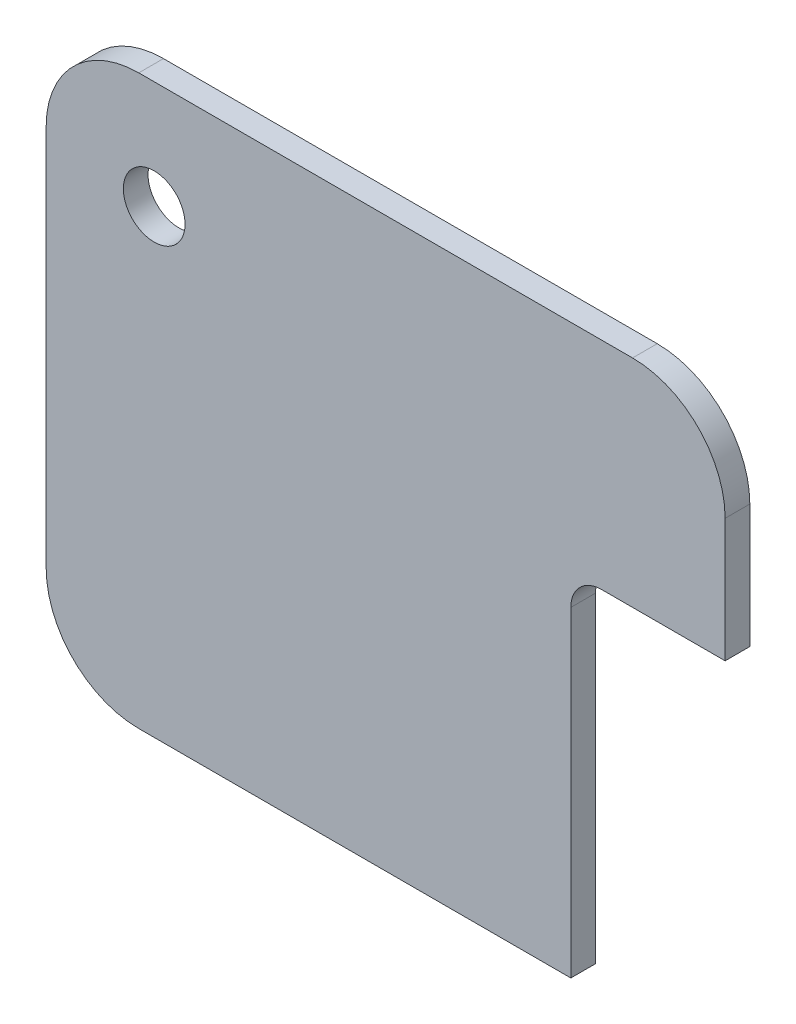
from build123d import *

# Parameters (mm, degrees)
SKETCH_1_R      = 10
EXTRUDE_1_DEPTH = 8


with BuildPart() as part:
    # 草图1 → 凸台-拉伸1 (new body)
    with BuildSketch(Plane.XY):
        with BuildLine():
            Line((0, 30), (0, 154))
            ThreePointArc((0, 154), (8.786796564, 175.213203436), (30, 184))
            Line((30, 184), (190, 184))
            ThreePointArc((190, 184), (211.213203436, 175.213203436), (220, 154))
            Line((220, 154), (220, 114))
            Line((220, 114), (180, 114))
            ThreePointArc((180, 114), (172.928932188, 111.071067812), (170, 104))
            Line((170, 104), (170, 0))
            Line((170, 0), (30, 0))
            ThreePointArc((30, 0), (8.786796564, 8.786796564), (0, 30))
        make_face()
        with Locations((35, 149)):
            Circle(SKETCH_1_R, mode=Mode.SUBTRACT)
    extrude(amount=EXTRUDE_1_DEPTH)


solid = part.part
